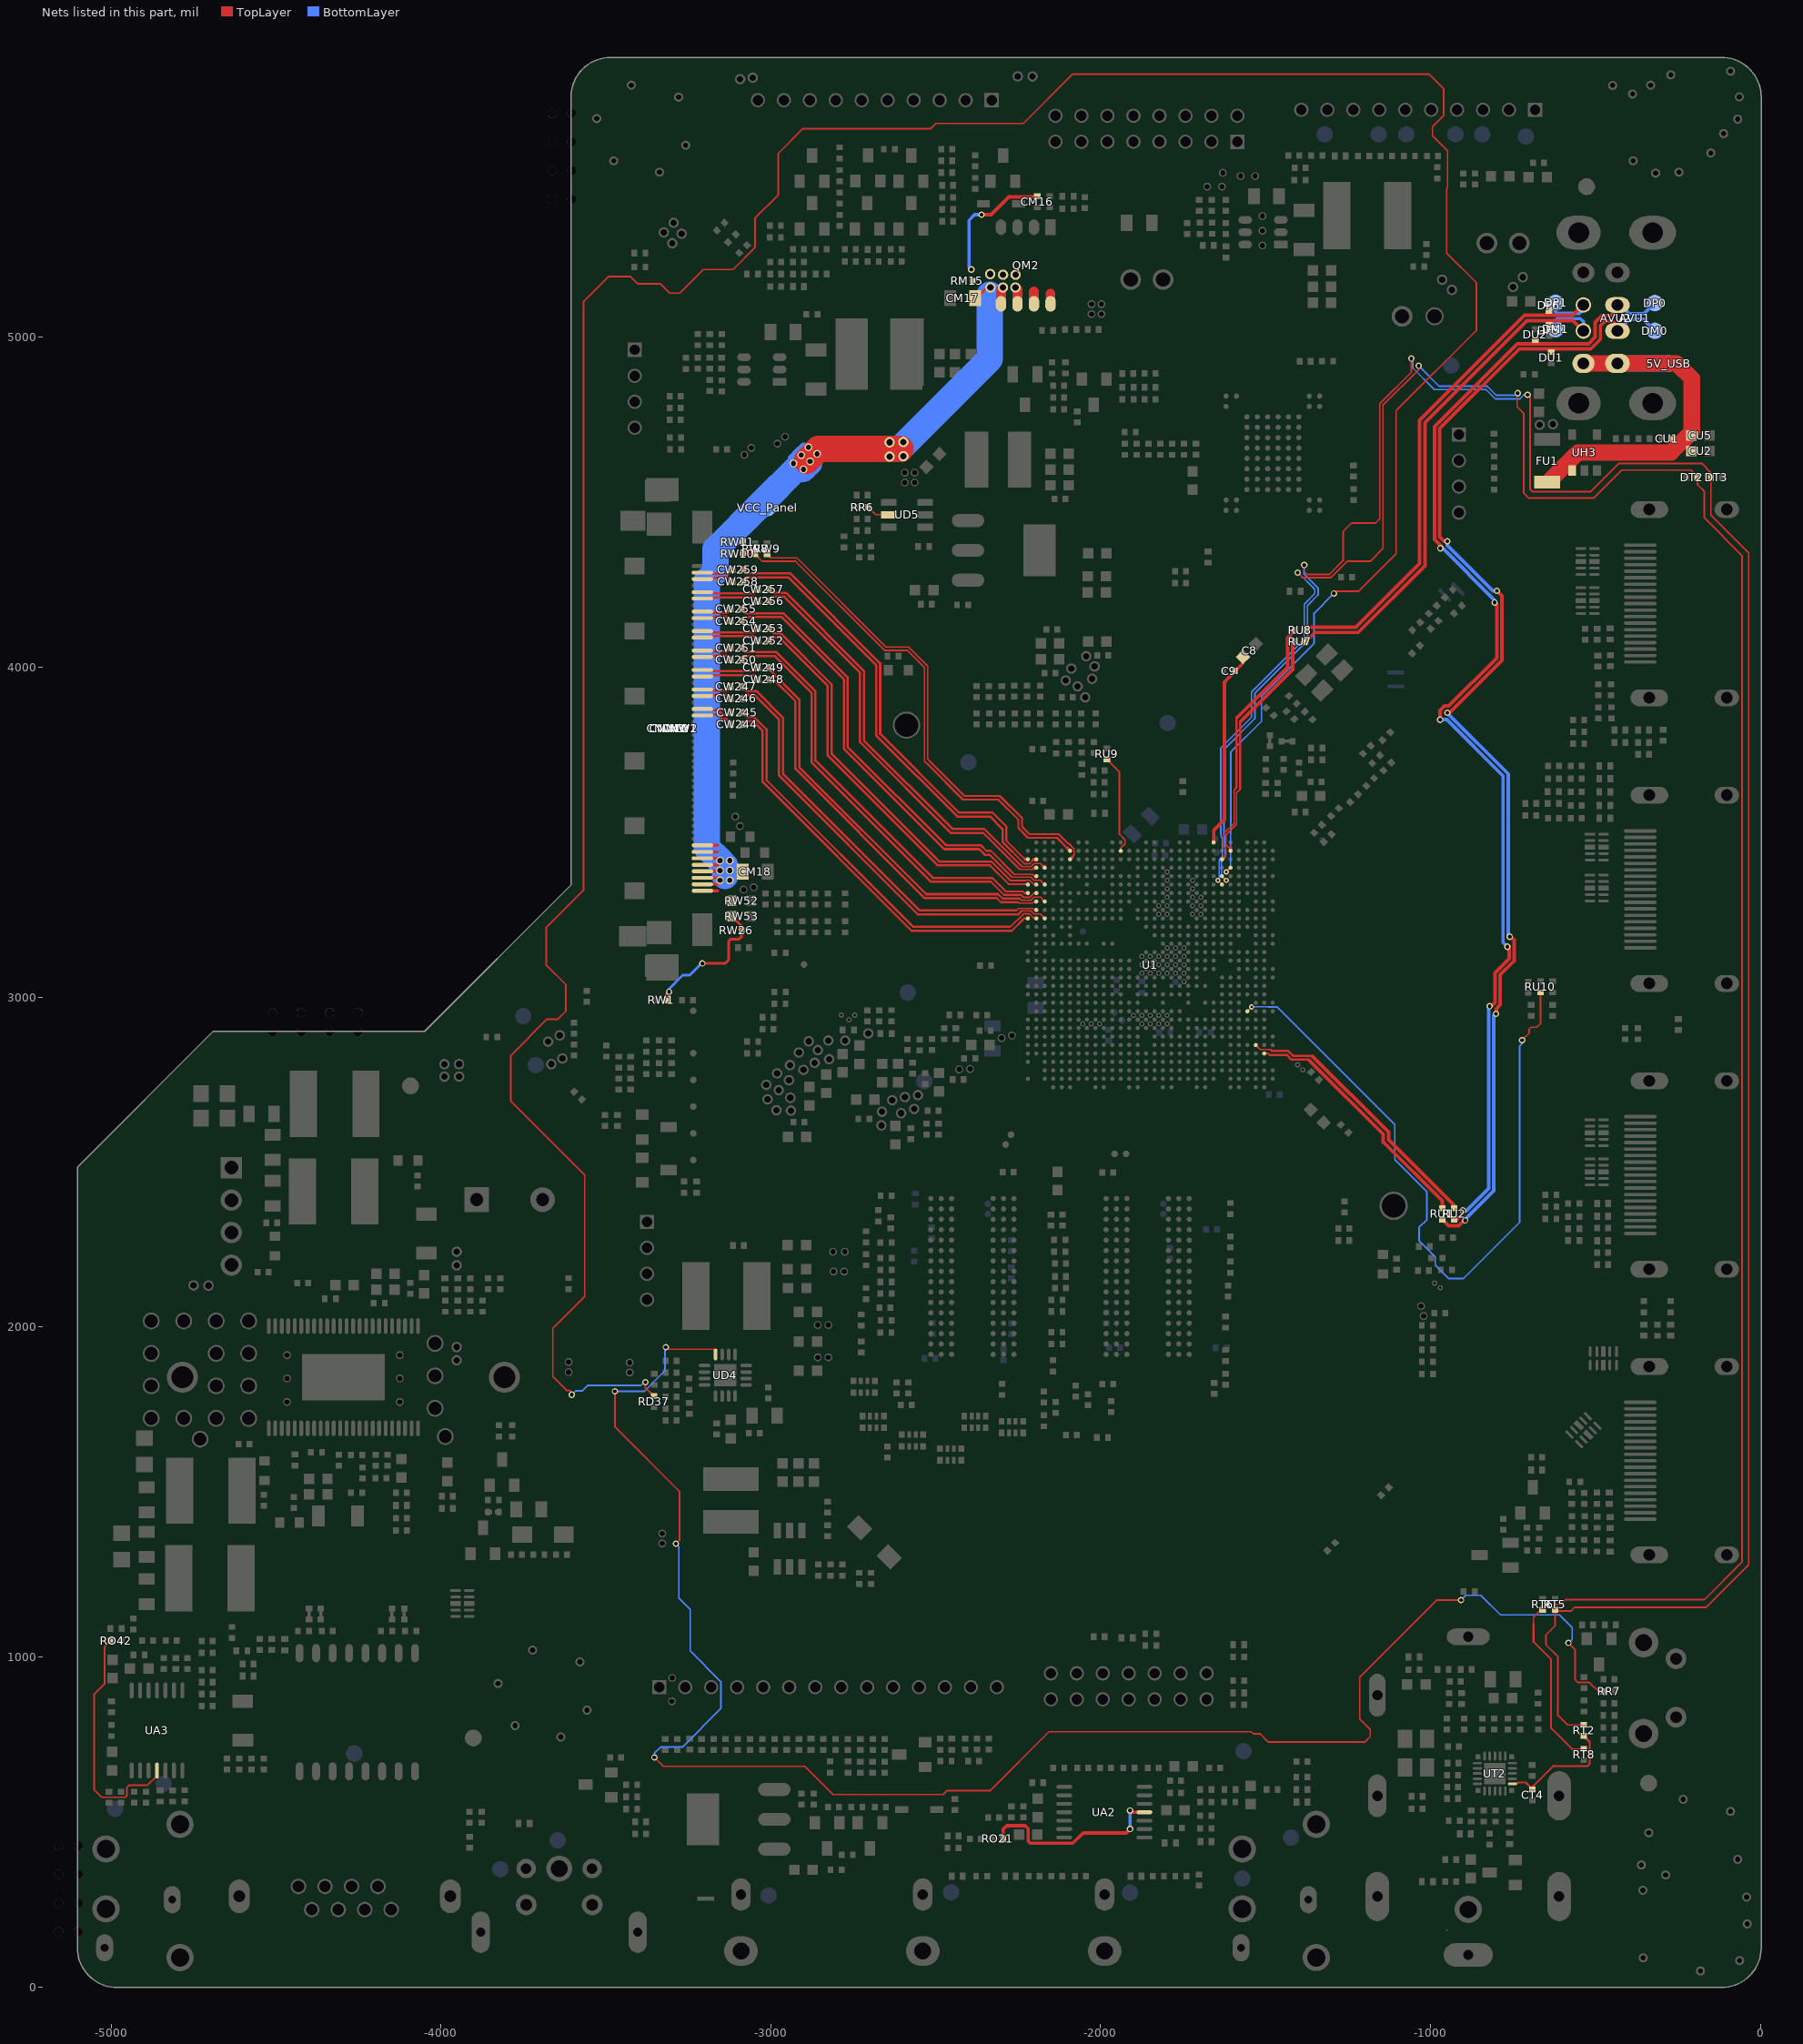
[diagram p0: the nets of this part, all layers, seen from the top]
# Altium PCB MISC86290.PcbDoc (part 28 of 31)
Units mil, origin at the board's own origin, x right, y up, seen from the top; angles counter-clockwise.
Board outline 5104.71 x 5851.49 mil, 2 copper layers (TopLayer, BottomLayer), stack 61.855 mil thick; 1026 components, 667 nets, 4280 pads, 2294 vias.

## Via types
v1: diameter 19.68, hole 11.81, TopLayer to BottomLayer, tented both sides, 1189 vias
v2: diameter 19.68/19.68 (per signal layer), hole 11.81, TopLayer to BottomLayer, tented both sides, 366 vias
v3: diameter 15.75, hole 7.87, TopLayer to BottomLayer, tented both sides, 348 vias
v4: diameter 23.62, hole 15.75, TopLayer to BottomLayer, tented both sides, 309 vias
v5: diameter 15.75/15.75 (per signal layer), hole 7.87, TopLayer to BottomLayer, tented both sides, 59 vias
v6: diameter 24/24 (per signal layer), hole 16, TopLayer to BottomLayer, tented both sides, 23 vias

## Nets (pads, with @x,y where several pads share a name; then routed paths per layer and width w, separated by ;. In a path a pad name is that pad's centre, name@x,y a point inside that pad or via, vN(x,y) a via of type N, cw(c..) or ccw(c..) an arc to the next point about the centre after c; other vN are vias at no path point) (continued)
TUNER_SCL_IC: DT2.K RT6.1 RT8.2 U1.AE7 | length 7748.2
  TopLayer w3.94: v3(-1645,3353.94) U1.AE7@-1632.2,3341.14
  TopLayer w5: v1(-1403,4287) -1387.45,4271.45 -1302.62,4271.45 -1252.8,4321.27 -1183.33,4321.27 -1144.25,4360.36 -1144.25,4794.65 -1036,4902.9 v1(-1036,4914) ; v1(-736,4831) -737.62,4829.38 -737.62,4789.67 -731.26,4783.31 ; -729.92,4781.97 -731.26,4783.31 ; -688,1099.5 -688,1120.77 RT6.1@-667,1141.77 ; RT6.1@-660.5,1142.43 -643.77,1159.15 -604.87,1159.15 -590.53,1173.5 -169.67,1173.5 -56,1287.17 -56,4338.86 -170,4452.86 -170,4533.14 -191.27,4554.41 DT2.K@-191.27,4576 ; DT2.K@-190.13,4577.13 -211,4598 -420.72,4598 -506.02,4512.7 -701.27,4512.7 -718,4529.43 -718,4770.05 -731.26,4783.31
  TopLayer w6: -688,1099.5 -688,1045.5 -634.5,992 -634.5,784 -570.73,720.23 RT8.2@-535.5,720.23
  BottomLayer w3.94: v3@-1641.06,3357.87 -1641.06,3415.99 -1630.94,3426.12 -1630.94,3482.44 -1635.53,3487.03 -1635.53,3493
  BottomLayer w5: -1635.95,3493 -1635.95,3755.26 -1542.74,3848.47 -1542.74,3925.04 -1383.04,4084.73 -1383.04,4191.43 -1351,4223.47 -1351,4236.53 -1401.47,4287 v1(-1403,4287) ; v1(-1036,4914) -974,4852 -828,4852 -800.76,4824.76 -742.24,4824.76 v1(-736,4831)
TUNER_SDA: CT4.1 RT2.1 UT2.2 | length 373.7
  TopLayer w6: UT2.2@-751.74,614.87 -739.36,614.87 -734.73,619.5 -712,619.5 -691,598.5 -691,605.85 -627.42,669.42 -627.14,669.14 -523.11,669.14 -517.5,674.75 -517.5,742 RT2.1@-535.5,760
TUNER_SDA_IC: DT3.K RT2.2 RT5.1 U1.AF7 | length 7757.4
  TopLayer w3.94: U1.AF7@-1632.2,3366.73 v3(-1619.41,3353.94)
  TopLayer w5: v1(-1383,4310) -1383,4291 -1373.45,4281.45 -1306.76,4281.45 -1265.26,4322.95 -1265.26,4411.1 -1239.22,4437.14 -1166.86,4437.14 -1154.25,4449.75 -1154.25,4798.79 -1058,4895.04 v1(-1058,4936) ; v1(-706,4826) -698,4818 -698,4539 -691.7,4532.7 -514.3,4532.7 -429,4618 -178,4618 -150,4590 -150,4461.14 -36,4347.14 -36,1278.89 -164.55,1150.34 -563.16,1150.34 -574.84,1138.66 -619.11,1138.66 RT5.1@-622.5,1142.05 -622.5,1094 -650,1066.5 -650,1036.49 -614,1000.49 -614,823 -584.46,793.46 RT2.2@-535.5,793.46
  BottomLayer w3.94: -1633.19,3412.5 -1633.19,3367.72 v3(-1619.41,3353.94) ; -1632.63,3412.5 -1622.5,3422.62 -1622.5,3487.06
  BottomLayer w5: -1623.54,3487.06 -1625.95,3489.48 -1625.95,3751.12 -1532.74,3844.33 -1532.74,3920.89 -1373.04,4080.59 -1373.04,4187.29 -1341,4219.33 -1341,4240.67 -1384,4283.67 v1@-1384,4309 ; v1@-1054,4936 -1054,4907.47 -988.53,4842 -832.14,4842 -803.8,4813.66 -728.82,4813.66 -716.47,4826
USB0_M: AVU1.2@-433.45,5019.67 AVU2.6 DM0.1 DU1.K RU1.2 | length 3671.8
  TopLayer w11: RU1.2@-964.6,2326.04 -945.23,2306.66 -914.14,2306.66 -897.8,2323 v1(-895,2323) ; v1(-949.26,4381.88) -958.88,4381.88 -972.25,4395.25 -972.25,4723.41 -730.65,4965 -634,4965 -514.25,4965 -485.25,4994 -485.25,5036 -471.25,5050 -449.25,5050 -434.69,5035.44 AVU1.2@-434.69,5019.67 ; v1(-949,3862) -942.83,3862 -783.5,4021.33 -783.5,4216.12 v1(-799,4231.62) ; v1(-801.5,2949.5) -800.66,2950.34 -800.66,2965.22 -789,2976.87 -789,3067.38 -746.34,3110.04 -746.34,3173.34 -756,3183 v1(-760,3183)
  BottomLayer w11: v1(-949.26,4381.88) -949.26,4369.26 -811.62,4231.62 v1(-799,4231.62) ; v1(-949,3862) -949,3861.43 -764.34,3676.77 -764.34,3187.34 v1(-760,3183) ; v1(-895,2323) -895,2326 -808.16,2412.84 ; -808.34,2413.03 -808.34,2909.5 ; -808.34,2915.24 -808.34,2909.5 ; v1(-801.5,2949.5) -808.34,2942.66 -808.34,2909.5 ; AVU1.2@-434.69,5019.67 AVU1.2@-433.45,5019.67 -398.11,5055 -355,5055 DM0.1@-320,5020 ; DM0.1@-324.5,5015.5 DM0.1@-319.5,5010.5
USB0_P: AVU1.3 AVU2.7 DP0.1 DU2.K RU2.2 | length 3582.2
  TopLayer w11: v2(-971,3841) -971,3868.77 -957.43,3882.34 -945.11,3882.34 -799.5,4027.96 v2@-799.5,4189.85 ; v2@-970.39,4369.39 -988.25,4387.25 -988.25,4730.03 -737.28,4981 -682.3,4981 -520.88,4981 -501.25,5000.63 -501.25,5045 -480.25,5066 -452.25,5066 -434.69,5083.55 AVU1.3@-434.69,5098.41 ; RU2.2@-928.33,2326.02 -920.75,2326.02 -902,2344.77 v2(-902,2353) ; v2@-816,2972.5 -805,2983.5 -805,3074.01 -762.34,3116.67 v2@-762.34,3153
  BottomLayer w11: v2(-971,3841) -951.2,3841 -780.34,3670.15 -780.34,3166.34 v2(-767,3153) ; v2@-963.38,4360.75 v2@-806,4203.37 ; v2(-902,2353) -891,2353 -824.34,2419.66 v2@-824.34,2969.16 ; AVU1.3@-434.69,5098.41 AVU1.3@-433.45,5098.41 -425,5098.41 -397.59,5071 -353,5071 DP0.1@-320,5104
  other v2: -821,2972.5 -806,4196.35 -970.39,4360.75
USB1_M: AVU2.2 DF5.K DM1.1 RU7.2 | length 1656.8
  TopLayer w11: RU7.2@-1378.27,4078 -1350.66,4105.61 -1219.39,4105.61 -1017.25,4307.75 -1017.25,4742.04 -708.29,5051 -569.18,5051 AVU2.2@-537.84,5019.67
  BottomLayer w10: DM1.1@-620.95,5024.72 -620.95,5052.05 -615.91,5057.09 -545.59,5057.09 -536.59,5048.09 AVU2.2@-536.59,5019.67
USB1_P: AVU2.3 DF6.K DP1.1 RU8.2 | length 1636.3
  TopLayer w11: RU8.2@-1378.27,4112 -1368.66,4121.61 -1226.02,4121.61 -1033.25,4314.38 -1033.25,4748.67 -714.92,5067 -569.25,5067 AVU2.3@-537.84,5098.41
  BottomLayer w11: DP1.1@-620.95,5105.12 -620.95,5076.45 -617.09,5072.59 -549.41,5072.59 -536.59,5085.41 AVU2.3@-536.59,5098.41
USB_5V: 5V_USB.1 AVU1.1@-433.45,4921.24 AVU2.1 AVU2.5 CU1.1 CU2.1 CU5.1 FU1.2 UH3.1 | length 1154.7
  TopLayer w50: FU1.2@-636.02,4568.02 -553.54,4650.5 -271.5,4650.5 -208,4714 -208,4875 -254.24,4921.24 AVU1.1@-433.45,4921.24 AVU2.1@-536.59,4921.24
  BottomLayer w50: AVU1.1@-434.69,4921.24 5V_USB.1@-277.25,4921.24
USB_EN: RU10.2 U1.K4 | length 2172.4
  TopLayer w5: U1.K4@-1555.43,2957.28 v3(-1542.64,2970.08) ; v1(-722.34,2869.73) -700.97,2891.1 -700.97,2902.82 -695.24,2908.55 -677.9,2908.55 -666.67,2919.77 -666.67,3013.94 RU10.2@-667,3014.27
  BottomLayer w5: v3@-1542.08,2970.63 -1491,2970.63 ; -1491,2970.53 -1465.75,2970.53 -1108.51,2613.3 -1108.51,2507.46 -1011,2409.94 -1011,2325.86 -1034.99,2301.87 -1034.99,2261.8 -985.66,2212.47 -985.66,2188.04 -944.27,2146.66 -900.99,2146.66 -729.68,2317.96 -729.68,2852 -722.34,2859.35 v1(-722.34,2869.73)
USB_OCN: RU9.1 U1.AJ19 | length 303.8
  TopLayer w3.94: U1.AJ19@-1939.29,3443.5 -1939.29,3451.38 -1925.59,3465.08 -1925.59,3476.7
  TopLayer w5: RU9.1@-1981.5,3720.77 -1943,3682.27 -1943,3494.11 -1927.22,3478.33
USB_P1_DM: RU1.1 U1.E2 | length 758.1
  TopLayer w5: U1.E2@-1504.25,2829.33 -1492.54,2829.33 -1488.16,2824.95
  TopLayer w6.8: -1488.16,2824.95 -1436.23,2824.95 -1421.97,2810.69 -1369.94,2810.69
  TopLayer w11: -1367.84,2808.59 -1143,2583.75 -1143,2561.13 -964.6,2382.73 RU1.1@-964.6,2359.5
USB_P1_DP: RU2.1 U1.F3 | length 825
  TopLayer w3.94: U1.F3@-1529.84,2854.92 -1516.65,2841.73 -1483.61,2841.73
  TopLayer w6.8: -1483.61,2840.22 -1480.14,2836.75 -1431.34,2836.75 -1417.08,2822.49 -1359.11,2822.49 -1357.01,2820.39
  TopLayer w11: -1357.01,2820.39 -1127,2590.38 -1127,2567.76 -928.33,2369.09 RU2.1@-928.33,2359.48
USB_P2_DM: RU7.1 U1.AJ6 | length 725.8
  TopLayer w3.94: U1.AJ6@-1607.11,3444 U1.AJ6@-1606.61,3443.5 ; U1.AJ6@-1607.11,3449.41 -1619.41,3461.71 -1619.41,3491.73 -1587.91,3523.23 -1587.91,3619.84 -1584.52,3623.23
  TopLayer w6: -1583.84,3623.92 -1577.47,3630.28 -1577.47,3833.65
  TopLayer w10: -1607.25,3453.19 -1606.61,3452.56 U1.AJ6@-1606.61,3443.5
  TopLayer w11: -1574.97,3836.15 -1417.5,3993.62 -1417.5,4072.23 RU7.1@-1411.73,4078
USB_P2_DP: RU8.1 U1.AH7 | length 791.9
  TopLayer w3.94: -1625.47,3424.65 -1619.41,3430.71 -1619.41,3448.43 -1627.28,3456.3 -1627.28,3495.67 -1595.79,3527.17 -1595.79,3627.57 -1592.37,3630.98
  TopLayer w5: -1592.37,3630.98 -1592.32,3631.03
  TopLayer w6: -1592.32,3631.03 -1588.47,3634.88 -1588.47,3845.28 -1585.97,3847.78
  TopLayer w10: U1.AH7@-1632.2,3417.91 -1625.47,3424.65
  TopLayer w11: -1585.97,3847.78 -1433.5,4000.25 -1433.5,4090.23 RU8.1@-1411.73,4112
UVP: RO42.2 UA3.11 | length 729.6
  TopLayer w5: RO42.2@-5001.89,1049 -5020,1030.89 -5020,917.18 -5051.67,885.5 -5051.67,597.67 -5028.31,574.31 -4956.8,574.31 -4952.41,578.7 -4952.41,603.5 -4944.91,611 -4889.5,611 -4860.92,639.58 UA3.11@-4860.92,655.21
UVP_HP: RO21.2 UA2.11 | length 582.5
  TopLayer w10: RO21.2@-2297.3,449 RO21.2@-2295.27,449 -2295.27,477.73 -2285,488 -2229.17,488 -2220,478.83 -2220,441.59 -2213.41,435 -2084.38,435 -2053.16,466.23 -1922.77,466.23 v1(-1911,478) ; v1(-1911,534) -1906,529 UA2.11@-1867.44,529
  BottomLayer w10: v1(-1911,478) v1(-1911,534)
VBY0N: CW244.1 U1.AA30 | length 1239.8
  TopLayer w6: -2269.25,3201.11 -2231.58,3238.78 U1.AA30@-2220.79,3238.78
  TopLayer w7: CW244.1@-3086.25,3824.62 -3073.87,3837 -3055.25,3837 -3024.75,3806.5 -3024.75,3652.55 -2573.31,3201.11 -2269.25,3201.11
VBY0N_2: CNW1.24 CNW2.24 CNW3.24 CNW12.24 CW244.2 | length 102.5
  TopLayer w7: CNW3.24@-3207.67,3853.9 -3175.35,3853.9 -3171.25,3858 -3163.17,3858 -3149.17,3844 -3136.71,3844 CW244.2@-3119.71,3827
VBY0P: CW245.1 U1.AA29 | length 1272.9
  TopLayer w5: -2274.51,3212.11 -2234.24,3252.38 -2215.07,3252.38 -2201.47,3238.78 U1.AA29@-2195.2,3238.78
  TopLayer w7: CW245.1@-3086.25,3863.46 -3071.79,3849 -3050.28,3849 -3012.75,3811.47 -3012.75,3657.52 -2568.34,3213.11 -2274.51,3213.11
VBY0P_2: CNW1.23 CNW2.23 CNW3.23 CNW12.23 CW245.2 | length 98.3
  TopLayer w7: CNW3.23@-3207.67,3873.58 -3177.8,3873.58 -3174.22,3870 -3158.2,3870 -3144.2,3856 -3127.17,3856 CW245.2@-3119.71,3863.46
VBY1N: CW246.1 U1.AA28 | length 1312.8
  TopLayer w3.94: -2241.79,3258.54 -2241.79,3259.76 -2240.14,3261.42 -2211.11,3261.42 -2201.27,3251.57 -2182.4,3251.57 U1.AA28@-2169.61,3238.78
  TopLayer w7: CW246.1@-3087.78,3905 -3076.78,3916 -3049.22,3916 -2975.25,3842.03 -2975.25,3672.34 -2553.51,3250.61 -2470,3250.61 -2250.95,3250.61 -2241.79,3259.76
VBY1N_2: CNW1.21 CNW2.21 CNW3.21 CNW12.21 CW246.2 | length 93.1
  TopLayer w7: CNW3.21@-3207.67,3912.95 -3175.35,3912.95 -3171.25,3917.05 -3133.3,3917.05 CW246.2@-3121.25,3905
VBY1P: CW247.1 U1.AB29 | length 1278
  TopLayer w3.94: -2255.5,3262.61 -2248.82,3269.29 -2206.02,3269.29 -2201.1,3264.37 U1.AB29@-2195.2,3264.37
  TopLayer w7: CW247.1@-3087.78,3941.45 -3074.33,3928 -3044.25,3928 -2963.25,3847 -2963.25,3677.31 -2548.54,3262.61 -2504,3262.61 -2255.5,3262.61
VBY1P_2: CNW1.20 CNW2.20 CNW3.20 CNW12.20 CW247.2 | length 93
  TopLayer w7: CNW3.20@-3207.67,3932.64 -3177.8,3932.64 -3174.22,3929.05 -3133.65,3929.05 CW247.2@-3121.25,3941.45
VBY2N: CW248.1 U1.AC29 | length 1213.8
  TopLayer w3.94: -2249.22,3286.53 -2247.73,3285.04 -2206.02,3285.04 -2201.1,3289.96 U1.AC29@-2195.2,3289.96
  TopLayer w6: -2315.07,3300.11 -2315,3300.11 -2302.67,3287.78 -2250.47,3287.78 -2249.22,3286.53
  TopLayer w7: CW248.1@-3005.83,3963.16 -2991.54,3963.16 -2925.75,3897.37 -2925.75,3692.14 -2533.72,3300.11 -2315.07,3300.11
VBY2N_2: CNW1.18 CNW2.18 CNW3.18 CNW12.18 CW248.2 | length 175.4
  TopLayer w7: CNW3.18@-3207.67,3972.01 -3175.35,3972.01 -3171.25,3976.11 -3052.25,3976.11 CW248.2@-3039.3,3963.16
VBY2P: CW249.1 U1.AC28 | length 1261.6
  TopLayer w3.94: -2240.72,3294.03 -2239.61,3292.91 -2211.93,3292.91 -2202.09,3302.76 -2182.4,3302.76 U1.AC28@-2169.61,3289.96
  TopLayer w6: -2311.47,3312.11 -2310.8,3312.11 -2297.47,3298.78 -2245.47,3298.78 -2240.72,3294.03
  TopLayer w7: CW249.1@-3005.85,3999.6 -3005.85,3994.43 -2913.75,3902.34 -2913.75,3697.11 -2528.75,3312.11 -2311.47,3312.11
VBY2P_2: CNW1.17 CNW2.17 CNW3.17 CNW12.17 CW249.2 | length 174.6
  TopLayer w7: CNW3.17@-3207.67,3991.69 -3177.8,3991.69 -3174.22,3988.11 -3050.8,3988.11 CW249.2@-3039.3,3999.61
VBY3N: CW250.1 U1.AD29 | length 1329
  TopLayer w5: -2235.12,3304.03 -2233.12,3302.03 -2215.72,3302.04 -2202.2,3315.55 U1.AD29@-2195.2,3315.55
  TopLayer w6: -2332.7,3349.61 -2292.87,3309.78 -2240.87,3309.78 -2235.12,3304.03
  TopLayer w7: CW250.1@-3087.78,4022.84 -3076.63,4034 -2988.28,4034 -2876.75,3922.46 -2876.75,3712.44 -2513.92,3349.61 -2432,3349.61 -2332.7,3349.61
VBY3N_2: CNW1.15 CNW2.15 CNW3.15 CNW12.15 CW250.2 | length 93.2
  TopLayer w7: CNW3.15@-3207.67,4031.06 -3175.35,4031.06 -3171.25,4035.16 -3133.57,4035.16 CW250.2@-3121.25,4022.84
VBY3P: CW251.1 U1.AD30 | length 1298.1
  TopLayer w6: -2329.1,3361.61 -2288.27,3320.78 -2236.27,3320.78 -2231.04,3315.55 U1.AD30@-2220.79,3315.55
  TopLayer w7: CW251.1@-3087.78,4059.3 -3074.49,4046 -2983.31,4046 -2864.75,3927.43 -2864.75,3717.41 -2508.95,3361.61 -2329.1,3361.61
VBY3P_2: CNW1.14 CNW2.14 CNW3.14 CNW12.14 CW251.2 | length 92.9
  TopLayer w7: CNW3.14@-3207.67,4050.75 -3177.8,4050.75 -3174.22,4047.16 -3133.38,4047.16 CW251.2@-3121.25,4059.3
VBY4N: CW252.1 U1.AE30 | length 1223.2
  TopLayer w6: -2336.07,3399.11 -2335.4,3399.11 -2279.07,3342.78 -2222.43,3342.78 U1.AE30@-2220.79,3341.14
  TopLayer w7: CW252.1@-3005.83,4081.16 -2995.99,4091 -2975.29,4091 -2827.75,3943.46 -2827.75,3732.73 -2494.13,3399.11 -2336.07,3399.11
VBY4N_2: CNW1.12 CNW2.12 CNW3.12 CNW12.12 CW252.2 | length 175.5
  TopLayer w7: CNW3.12@-3207.67,4090.12 -3175.35,4090.12 -3171.25,4094.22 -3052.36,4094.22 CW252.2@-3039.3,4081.16
VBY4P: CW253.1 U1.AE29 | length 1256.1
  TopLayer w5: -2228.4,3353.78 -2227.89,3354.29 -2215.24,3354.29 -2202.09,3341.14 U1.AE29@-2195.2,3341.14
  TopLayer w6: -2335.49,3411.11 -2331.8,3411.11 -2274.47,3353.78 -2228.4,3353.78
  TopLayer w7: CW253.1@-3005.83,4117.61 -2991.22,4103 -2970.32,4103 -2815.75,3948.43 -2815.75,3737.7 -2489.16,3411.11 -2335.49,3411.11
VBY4P_2: CNW1.11 CNW2.11 CNW3.11 CNW12.11 CW253.2 | length 174.6
  TopLayer w7: CNW3.11@-3207.67,4109.8 -3177.8,4109.8 -3174.22,4106.22 -3050.69,4106.22 CW253.2@-3039.3,4117.61
VBY5N: CW254.1 U1.AE28 | length 1382.4
  TopLayer w3.94: -2270.92,3365.83 -2268.87,3363.78 -2211.93,3363.78 -2202.09,3353.94 -2182.4,3353.94 U1.AE28@-2169.61,3341.14
  TopLayer w6: -2337.53,3432.11 -2337.2,3432.11 -2270.92,3365.83
  TopLayer w7: CW254.1@-3087.78,4140.38 -3076.17,4152 -2966.99,4152 -2778.75,3963.75 -2778.75,3753.03 -2474.33,3448.61 -2368.5,3448.61 -2351.67,3431.78 -2337.53,3431.78
VBY5N_2: CNW1.9 CNW2.9 CNW3.9 CNW12.9 CW254.2 | length 93.5
  TopLayer w7: CNW3.9@-3207.67,4149.17 -3175.35,4149.17 -3171.25,4153.27 -3134.14,4153.27 CW254.2@-3121.25,4140.39
VBY5P: CW255.1 U1.AF29 | length 1351.6
  TopLayer w3.94: -2263.12,3373.63 -2261.15,3371.65 -2206.02,3371.65 -2201.1,3366.73 U1.AF29@-2195.2,3366.73
  TopLayer w6: -2333.93,3443.78 -2333.27,3443.78 -2263.12,3373.63
  TopLayer w7: CW255.1@-3087.78,4176.84 -3074.94,4164 -2962.02,4164 -2766.75,3968.72 -2766.75,3758 -2469.36,3460.61 -2363.53,3460.61 -2346.7,3443.78 -2333.93,3443.78
VBY5P_2: CNW1.8 CNW2.8 CNW3.8 CNW12.8 CW255.2 | length 92.7
  TopLayer w7: CNW3.8@-3207.67,4168.86 -3177.8,4168.86 -3174.22,4165.27 -3132.82,4165.27 CW255.2@-3121.25,4176.84
VBY6N: CW256.1 U1.AG29 | length 1283.7
  TopLayer w3.94: -2247.52,3389.23 -2245.69,3387.4 -2206.02,3387.4 -2202.23,3391.19
  TopLayer w6: -2357.07,3498.11 -2356.4,3498.11 -2247.52,3389.23
  TopLayer w7: CW256.1@-3005.83,4200.33 -2992.16,4214 -2959.7,4214 -2729.75,3984.05 -2729.75,3773.33 -2454.53,3498.11 -2357.07,3498.11
  TopLayer w10: -2201.44,3390.4 -2199.51,3392.32 U1.AG29@-2195.2,3392.32
VBY6N_2: CNW1.6 CNW2.6 CNW3.6 CNW12.6 CW256.2 | length 175
  TopLayer w7: CNW3.6@-3207.67,4208.23 -3175.35,4208.23 -3171.25,4212.33 -3051.29,4212.33 CW256.2@-3039.3,4200.33
VBY6P: CW257.1 U1.AG28 | length 1317.6
  TopLayer w3.94: -2239.72,3397.03 -2237.97,3395.28 -2211.93,3395.28 -2202.09,3405.12 -2182.4,3405.12 U1.AG28@-2173.72,3396.44
  TopLayer w6: -2353.37,3510.11 -2352.8,3510.11 -2239.72,3397.03
  TopLayer w7: CW257.1@-3005.83,4236.79 -2995.04,4226 -2954.73,4226 -2717.75,3989.02 -2717.75,3778.3 -2449.56,3510.11 -2353.37,3510.11
  TopLayer w10: U1.AG28@-2173.72,3396.44 U1.AG28@-2169.61,3392.32
VBY6P_2: CNW1.5 CNW2.5 CNW3.5 CNW12.5 CW257.2 | length 175
  TopLayer w7: CNW3.5@-3207.67,4227.91 -3177.8,4227.91 -3174.22,4224.33 -3051.76,4224.33 CW257.2@-3039.3,4236.79
VBY7N: CW258.1 U1.AH29 | length 1406
  TopLayer w5: -2233.27,3406.18 -2231.81,3404.72 -2215.04,3404.72 -2204.25,3415.5
  TopLayer w6: -2297.69,3471.27 -2297.69,3470.6 -2233.27,3406.18
  TopLayer w7: CW258.1@-3082.52,4259.84 -3069.36,4273 -2946.98,4273 -2680.75,4006.76 -2680.75,3793.62 -2434.74,3547.61 -2335.5,3547.61 -2297.69,3509.81 -2297.69,3471.27
  TopLayer w10: -2204.74,3415.99 -2202.81,3417.91 U1.AH29@-2195.2,3417.91
VBY7N_2: CNW1.3 CNW2.3 CNW3.3 CNW12.3 CW258.2 | length 98.2
  TopLayer w7: CNW3.3@-3207.67,4267.28 -3175.35,4267.28 -3171.25,4271.38 -3127.52,4271.38 CW258.2@-3115.98,4259.84
VBY7P: CW259.1 U1.AH30 | length 1375.8
  TopLayer w6: -2285.69,3474.87 -2285.69,3474.2 -2229.41,3417.91 -2229.12,3417.91
  TopLayer w7: CW259.1@-3082.52,4296.3 -3071.22,4285 -2942.01,4285 -2668.75,4011.73 -2668.75,3798.59 -2429.77,3559.61 -2328.5,3559.61 -2285.69,3516.81 -2285.69,3474.87
  TopLayer w10: -2229.12,3418.86 -2228.18,3417.91 U1.AH30@-2220.79,3417.91
VBY7P_2: CNW1.2 CNW2.2 CNW3.2 CNW12.2 CW259.2 | length 98.5
  TopLayer w7: CNW3.2@-3207.67,4286.97 -3177.8,4286.97 -3174.22,4283.38 -3128.89,4283.38 CW259.2@-3115.98,4296.3
VBY_HTPDN: RW9.2 RW11.2 U1.AH25 | length 1608.2
  TopLayer w3.94: -2089.88,3459.25 -2080.04,3449.41 -2080.04,3430.71 -2086.25,3424.5
  TopLayer w5: RW11.2@-3084.25,4380 -3084.25,4379.25 -3064,4359 -3027.5,4359 -3011.5,4343 RW9.2@-3011.5,4342.27 -3000.73,4331.5 -2921.13,4331.5 -2650.98,4061.34 -2582.2,4061.34 -2524.5,4003.64 -2524.5,3721.52 -2519.75,3716.77
  TopLayer w6: RW11.2@-3084.52,4380.27 RW11.2@-3084.25,4380 ; -2519.75,3716.77 -2413.09,3610.11 -2306,3610.11 -2238.19,3542.31 -2238.19,3516.35 -2215.85,3494 -2127.77,3494 -2099.21,3465.43 -2096.38,3465.43 -2095.36,3464.41 -2095.04,3464.41 -2089.88,3459.25
  TopLayer w10: U1.AH25@-2092.83,3417.91 -2086.25,3424.5
VBY_LOCKN: RW8.2 RW10.2 U1.AJ25 | length 1540.3
  TopLayer w5: RW8.2@-3047.5,4342.27 -3026.73,4321.5 -2925.27,4321.5 -2655.12,4051.34 -2586.34,4051.34 -2534.5,3999.5 -2534.5,3715.96 -2524.77,3706.23
  TopLayer w6: RW10.2@-3084.05,4344 RW8.2@-3052,4344 ; -2524.77,3706.23 -2417.65,3599.11 -2310.56,3599.11 -2249.19,3537.75 -2249.19,3511.79 -2220.41,3483 -2132.33,3483 -2101.76,3452.43
  TopLayer w10: -2101.76,3452.43 U1.AJ25@-2092.83,3443.5
VCC_PANEL: CM16.2 CM17.1 CM18.1 CNW1.44 CNW1.45 CNW1.46 CNW1.47 CNW1.48 CNW1.49 CNW1.50 CNW1.51 CNW2.44 CNW2.45 CNW2.46 CNW2.47 CNW2.48 CNW2.49 CNW2.50 CNW2.51 CNW3.44 CNW3.45 CNW3.46 CNW3.47 CNW3.48 CNW3.49 CNW3.50 CNW3.51 CNW12.44 CNW12.45 CNW12.46 CNW12.47 CNW12.48 CNW12.49 CNW12.50 CNW12.51 pad.VIA5@-2258,5190 pad.VIA5@-2258.35,5151.26 pad.VIA5@-2296,5190 pad.VIA5@-2296.35,5151.26 pad.VIA5@-2334.35,5151.26 pad.VIA5@-2335,5192 pad.VIA5@-2598,4640 pad.VIA5@-2598,4683 pad.VIA5@-2640,4639 pad.VIA5@-2640,4682 pad.VIA5@-2860,4647 pad.VIA5@-2881,4624 pad.VIA5@-2886,4667 pad.VIA5@-2901,4600 pad.VIA5@-2908,4643 pad.VIA5@-2931,4618 pad.VIA5@-3124.25,3354 pad.VIA5@-3124.25,3384 pad.VIA5@-3124.25,3414 pad.VIA5@-3154.25,3354 pad.VIA5@-3154.25,3384 pad.VIA5@-3154.25,3414 QM2.5 QM2.6 QM2.7 QM2.8 RM15.1 RW1.2 RW26.2 RW52.1 RW53.1 VCC_Panel.1 | length 3796
  TopLayer w5: CM17.1@-2372.52,5125 CM17.1@-2368.52,5129
  TopLayer w8: RW1.2@-3316.27,2991 -3316.27,3008.23 v1(-3308.5,3016) ; v1(-3207.5,3102) -3139,3102 -3128,3113 -3128,3169.5 -3121.5,3176 -3096,3176 -3088.77,3183.23 RW26.2@-3088.77,3202 -3088.77,3215.49 RW53.1@-3118.28,3245
  TopLayer w9: CNW3.51@-3207.67,3322.4 -3161.25,3322.4 ; CNW3.50@-3207.67,3342.09 -3161.25,3342.09 ; CNW3.49@-3207.67,3361.77 pad.VIA5@-3161.25,3361.77 ; CNW3.48@-3207.67,3381.46 pad.VIA5@-3161.25,3381.46 ; CNW3.47@-3207.67,3401.14 -3161.25,3401.14 ; CNW3.46@-3207.67,3420.83 pad.VIA5@-3161.25,3420.83 ; CNW3.45@-3207.67,3440.51 -3161.25,3440.51 ; CNW3.44@-3207.67,3460.2 -3161.25,3460.2
  TopLayer w10: CM17.1@-2368.52,5129 -2367.25,5129 pad.VIA5@-2342.56,5153.69 ; v1@-2360.05,5370.55 v1(-2361.5,5372) -2332.25,5372 -2278.42,5425.83 -2194.15,5425.83 CM16.2@-2192.25,5427.73
  TopLayer w30: QM2.5@-2302.25,5101.86 -2302.25,5145.36 pad.VIA5@-2296.35,5151.26 ; pad.VIA5@-2258.35,5151.26 -2252.25,5145.16 QM2.6@-2252.25,5101.86 ; QM2.7@-2202.25,5101.86 -2202.25,5139 ; QM2.8@-2152.25,5101.86 -2152.25,5132
  TopLayer w80: pad.VIA5@-2890.83,4626.16 -2887,4630 -2868,4649 -2865,4652 -2855.64,4661.35 -2640,4661.35 -2607,4661.35
  BottomLayer w8: v1(-3308.5,3016) -3312,3019.5 -3312,3021.27 -3266.77,3066.5 -3246,3066.5 -3210.5,3102 v1(-3207.5,3102)
  BottomLayer w10: v1(-2392.12,5206.12) -2399.5,5213.5 -2399.5,5334 -2399.5,5355.27 -2382.77,5372 v1(-2361.5,5372)
  BottomLayer w30: -2933.99,4605.33 pad.VIA5@-2933.99,4608.22 ; -2933.99,4632.49 -2915.74,4650.74 -2899.74,4666.74 ; pad.VIA5@-2879.74,4666.74 pad.VIA5@-2860,4647
  BottomLayer w80: -3138.25,3367 -3138.25,3384 -3138.25,3398 -3139.25,3399 pad.VIA5@-3154.25,3414 -3193.61,3453.36 -3193.61,4263.27 -3167.25,4289.63 -3167.25,4357.93 -3025.79,4499.39 -2919.09,4606.09 -2913.09,4612.09 -2912.84,4612.34 ; pad.VIA5@-2902.48,4601.48 pad.VIA5@-2884.48,4619.48 ; -2628,4661.35 -2609.65,4661.35 -2593,4678 -2336.25,4934.75 -2336.25,5130
VDDC_CAP: C8.2 C9.1 U1.AK8 | length 599.2
  TopLayer w10: U1.AK8@-1657.8,3469.09 -1657.8,3504.96 -1624.72,3538.03 -1624.72,3955.59 -1568.67,4011.65 C8.2@-1568.67,4031.33
VDDC_PGOOD: RR7.2 UD4.4 | length 5351.8
  TopLayer w5: v1(-3473,1805) -3473,1697.69 -3277,1501.69 -3277,1354 v1(-3288,1343) ; v1(-3353,695) -3326.18,668.18 -3183.26,668.18 -2897.01,668.18 -2811.17,582.34 -2477.91,582.34 -2466.25,594 ; v1@-3318.5,1932.5 -3174.5,1932.5 -3167.54,1925.54 UD4.4@-3167.54,1916.68 ; -2465.14,594 -2336.12,594 -2157.12,773 -1543.75,773 -1537.5,766.75 -1516.72,766.75 -1491.47,741.5 -1199.83,741.5 -1183,758.33 -1183,779.67 -1214.49,811.15 -1214.49,937.97 -980.27,1172.18 v1(-907.5,1172.18) ; v2(-582,1042) -562,1022 -562,932 -552.37,922.37 -518.41,922.37 -491.19,895.16 RR7.2@-475.73,895.16
  BottomLayer w5: v1(-3473,1805) -3383.21,1805 -3321,1867.21 v1@-3321,1939 ; v1(-3353,695) -3353,707.5 -3334,726.5 -3268.21,726.5 -3151.56,843.16 -3151.56,895.86 ; v1(-3288,1343) -3278.75,1333.75 -3278.75,1201 -3278.75,1178.53 -3244.25,1144.03 -3244.25,1017.75 -3151.56,925.06 -3151.56,920.14 ; -3151.49,895.92 -3151.49,920.08 ; v1(-907.5,1172.18) -893.34,1186.34 -847.34,1186.34 -788,1127 -609,1127 -570.87,1088.87 -570.87,1053.13 v2(-582,1042)
  other v1: -3318.5,1939
VDDCPU_PGOOD: RR6.2 UD5.5 | length 73.9
  TopLayer w5: RR6.2@-2706.7,4485 -2704.5,4485 -2682,4462.5 UD5.5@-2642.12,4462.5
VID0: RD37.1 U1.AG6 | length 9819.9
  TopLayer w3.94: v3(-1619.41,3379.53) U1.AG6@-1606.61,3392.32
  TopLayer w5: v1@-3603.34,1800.34 -3610.31,1807.31 -3618.49,1807.31 -3661,1849.82 -3661,1995.42 -3564.25,2092.17 -3564.25,2460.54 -3788,2684.29 -3788,2823.35 -3678.35,2933 -3645.66,2933 -3621.5,2957.16 -3621.5,3037.86 -3681,3097.36 -3681,3210.34 -3568.11,3323.23 -3568.11,5108.42 -3491.53,5185 -3425.91,5185 -3403.25,5162.34 -3333.77,5162.34 -3305.93,5134.5 -3276.35,5134.5 -3204.85,5206 -3114.14,5206 -3048.09,5272.05 -3048.09,5361.19 -2978,5431.28 -2978,5556.79 -2901.94,5632.85 -2514.94,5632.85 -2499.28,5648.5 -2234.28,5648.5 -2084.33,5798.46 -1004.92,5798.46 -960.04,5753.57 -960.04,5673.02 -994,5639.06 -994,5611.14 -948.61,5565.75 -948.61,5454.89 -951.53,5451.96 -951.53,5256.08 -861.09,5165.64 -861.09,5021.24 -1104.25,4778.08 -1104.25,4343.79 -1217.32,4230.72 -1286.28,4230.72 v1(-1293,4224) ; v1(-3380.16,1832.57) -3381,1831.73 -3381,1816.73 RD37.1@-3354.5,1790.23
  BottomLayer w3.94: v3@-1618.43,3380.64 -1605.63,3393.45 -1605.63,3499.18
  BottomLayer w5: v1(-3603.34,1794.77) -3592.12,1806 -3572,1806 -3555.48,1822.52 -3393.89,1822.52 -3382,1834.42 v1(-3380.16,1832.57) ; -1605.95,3499.18 -1605.95,3742.84 -1512.74,3836.05 -1512.74,3912.61 -1353.04,4072.31 -1353.04,4163.96 v1(-1293,4224)